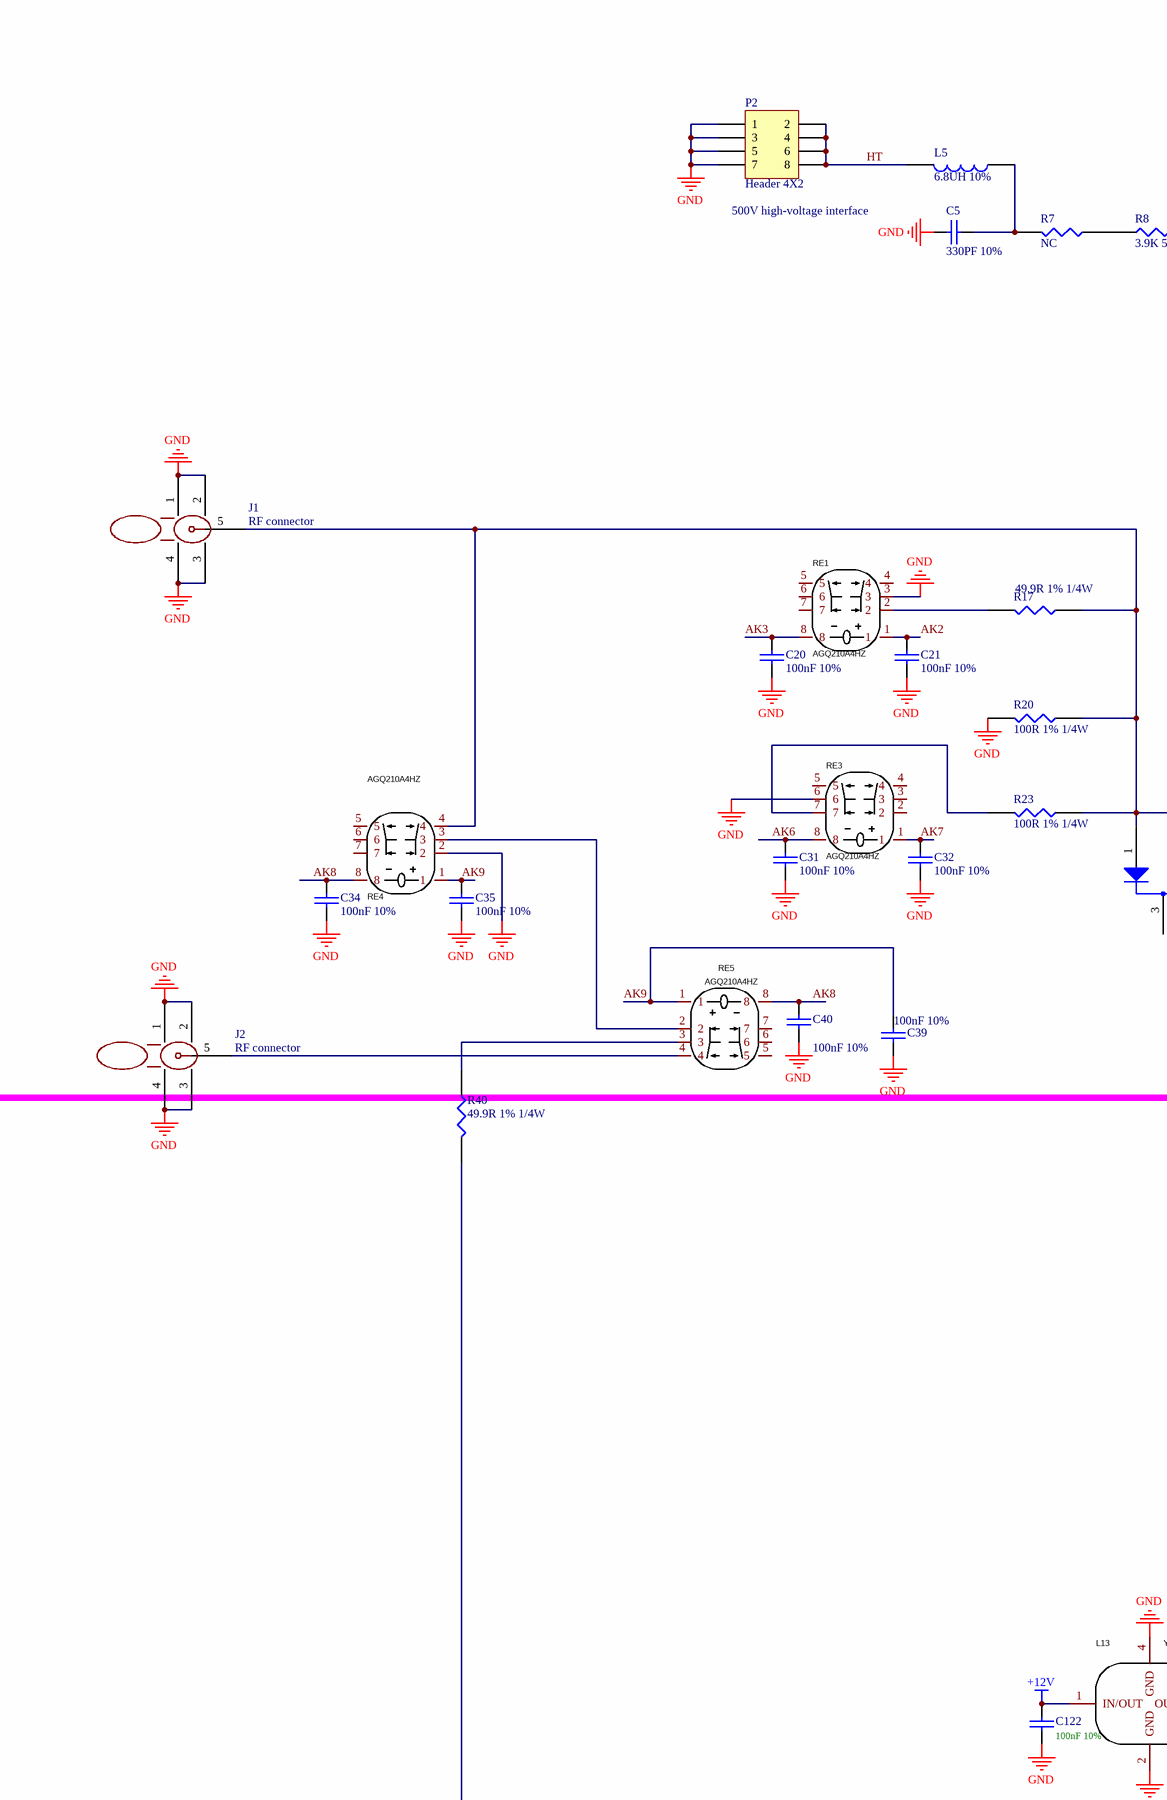
[diagram p0: PCBE109560-10.SchDoc, top left]
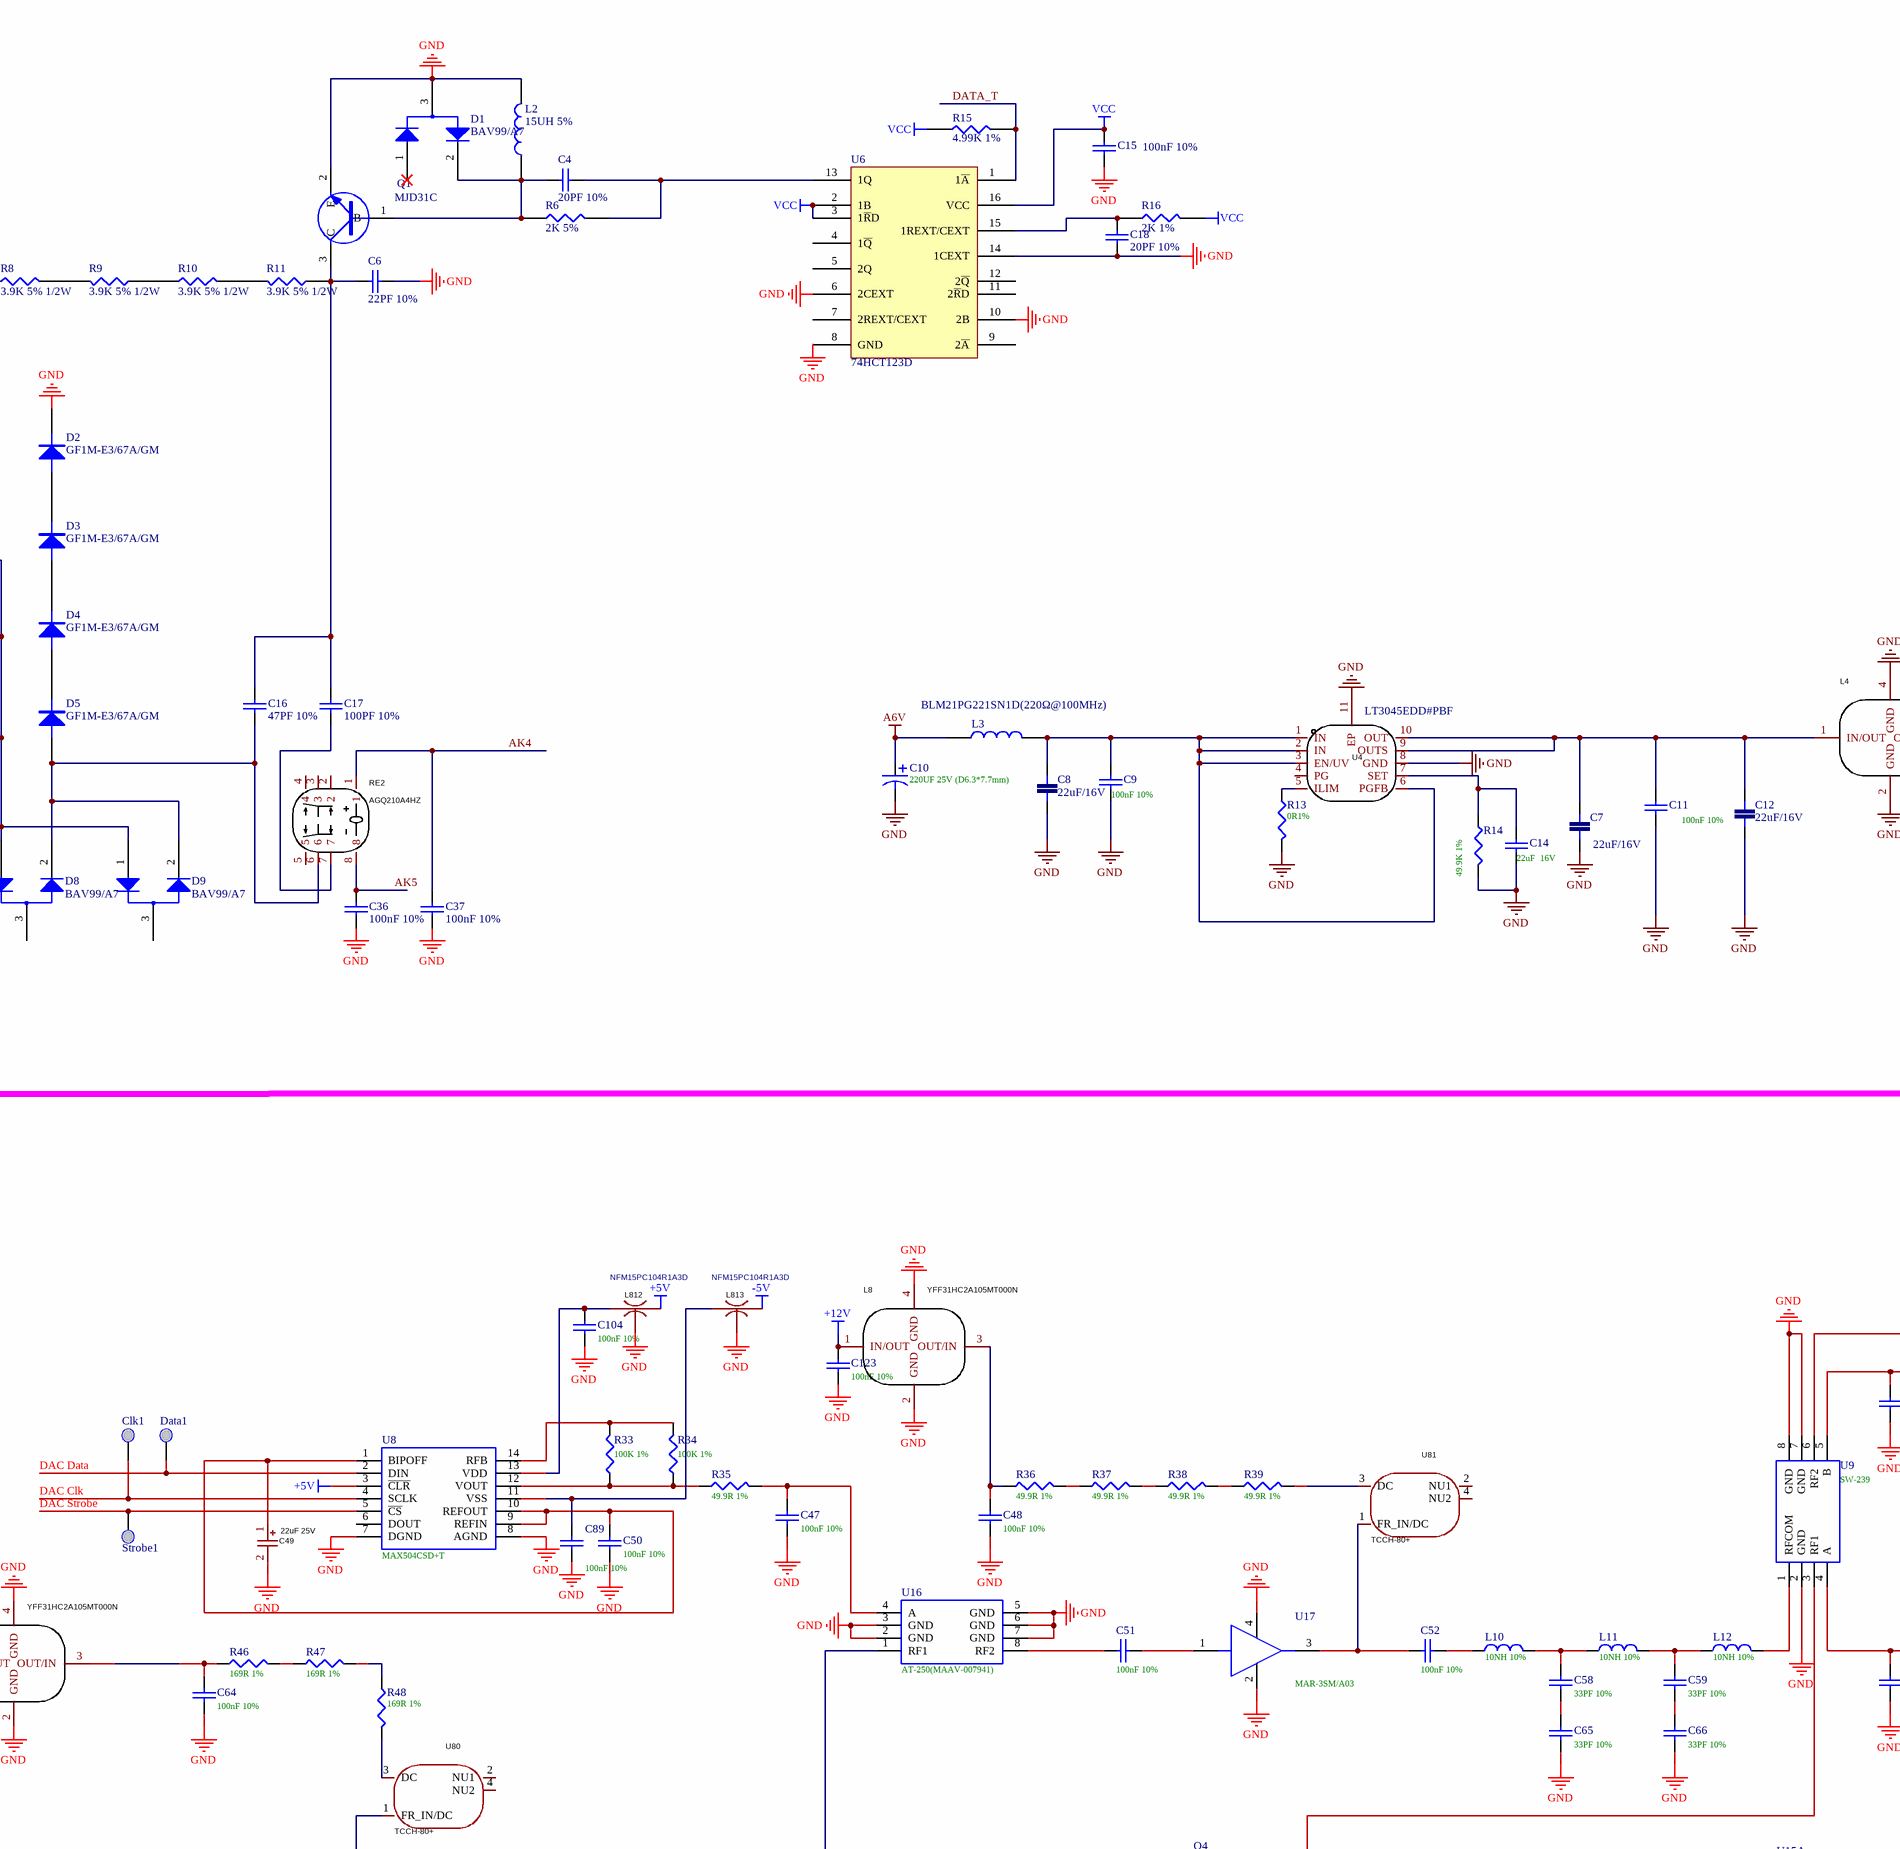
[diagram p1: PCBE109560-10.SchDoc, top middle]
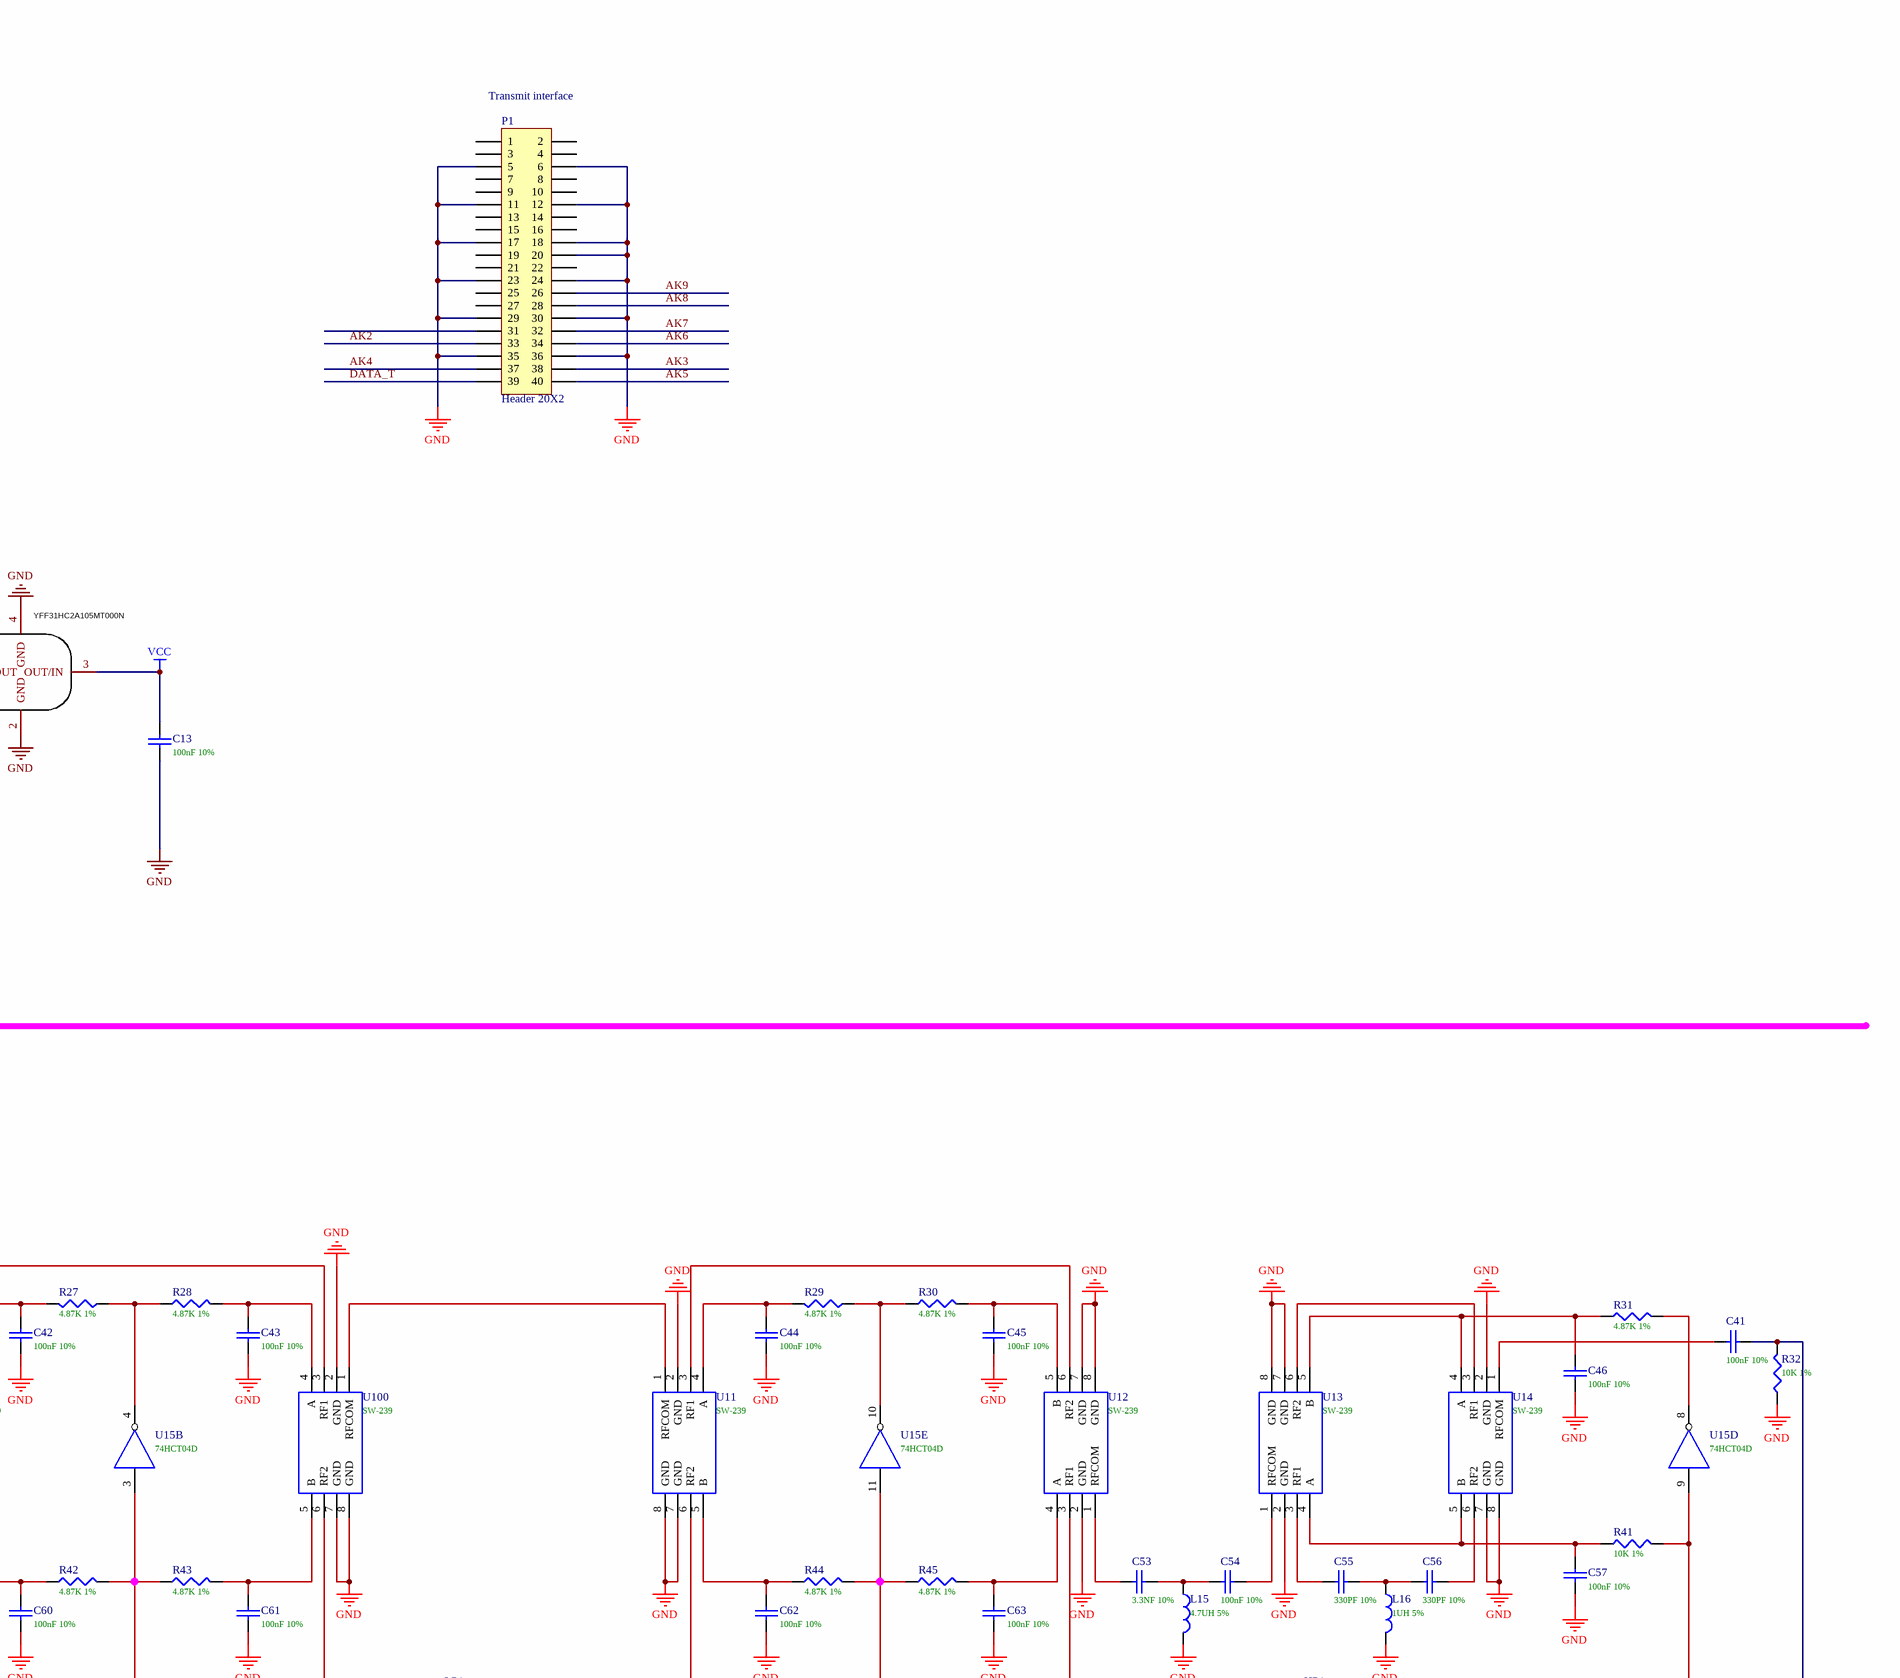
[diagram p2: PCBE109560-10.SchDoc, top right]
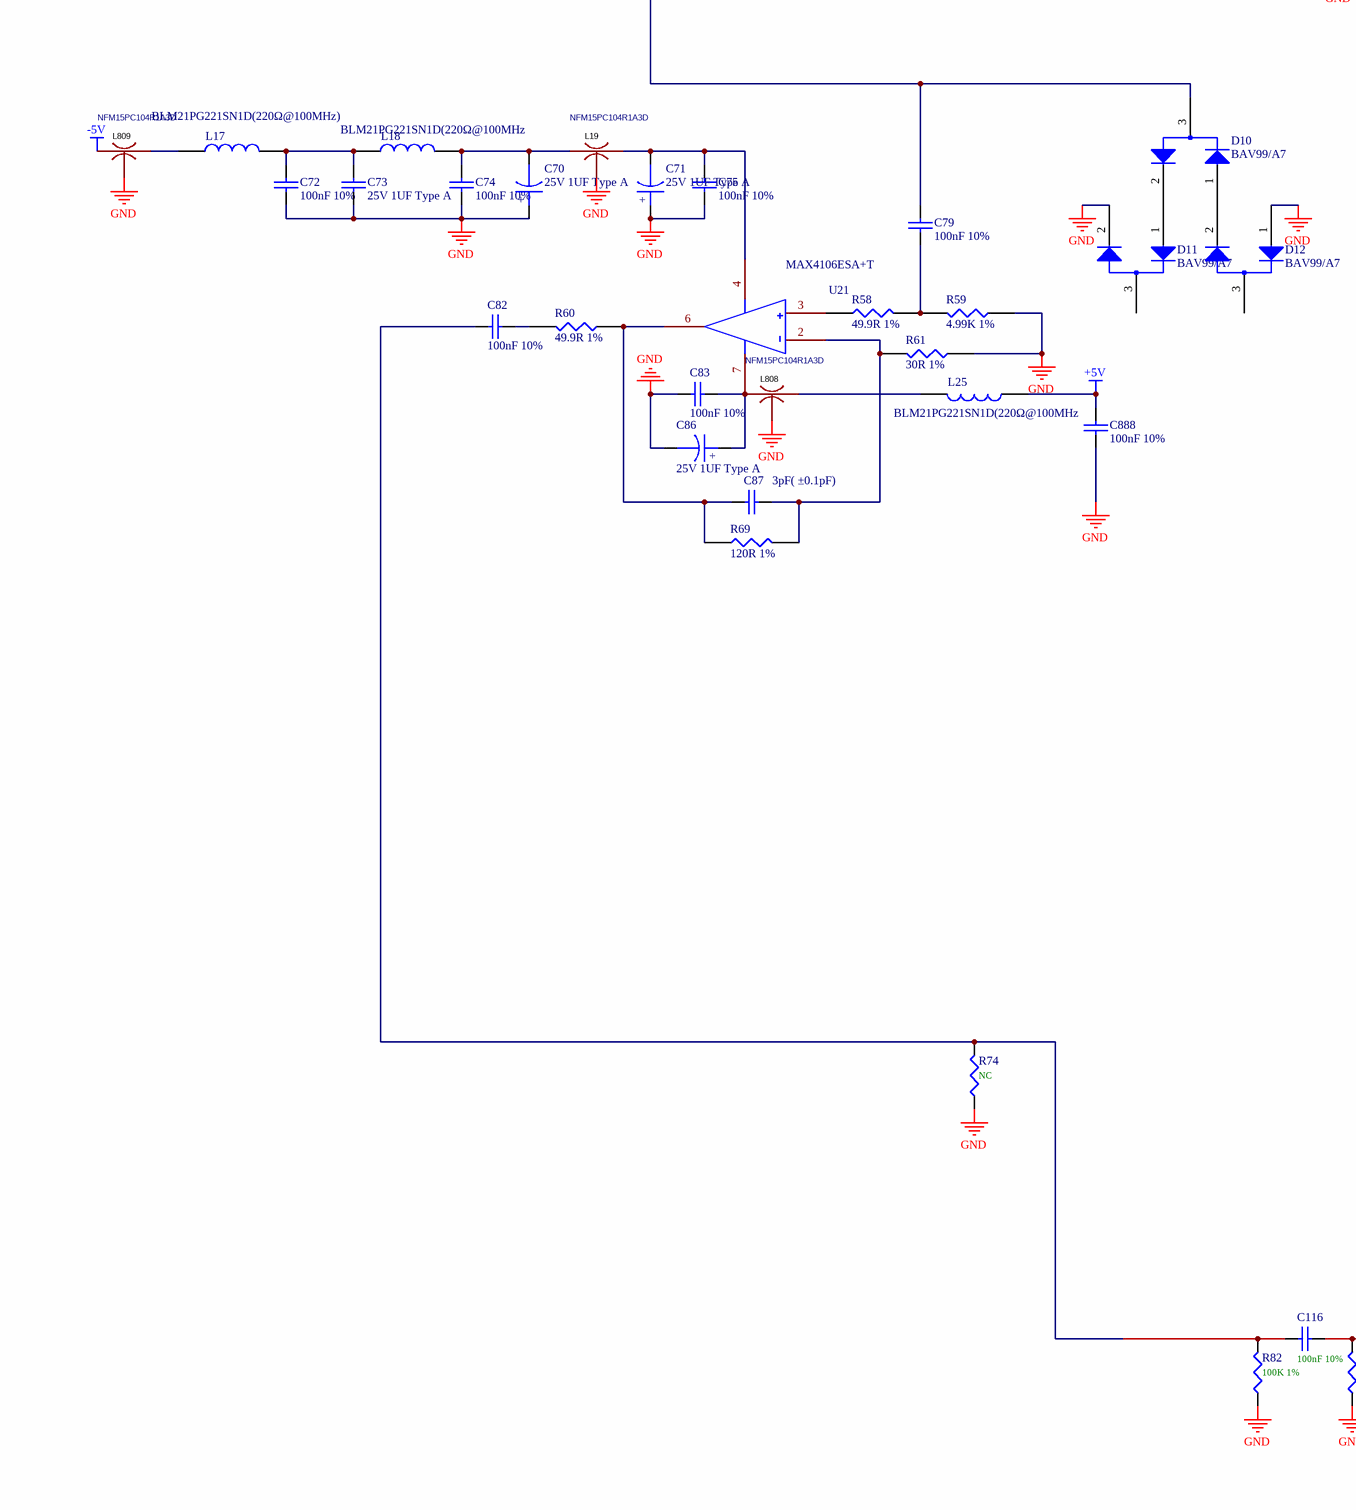
[diagram p3: PCBE109560-10.SchDoc, bottom left]
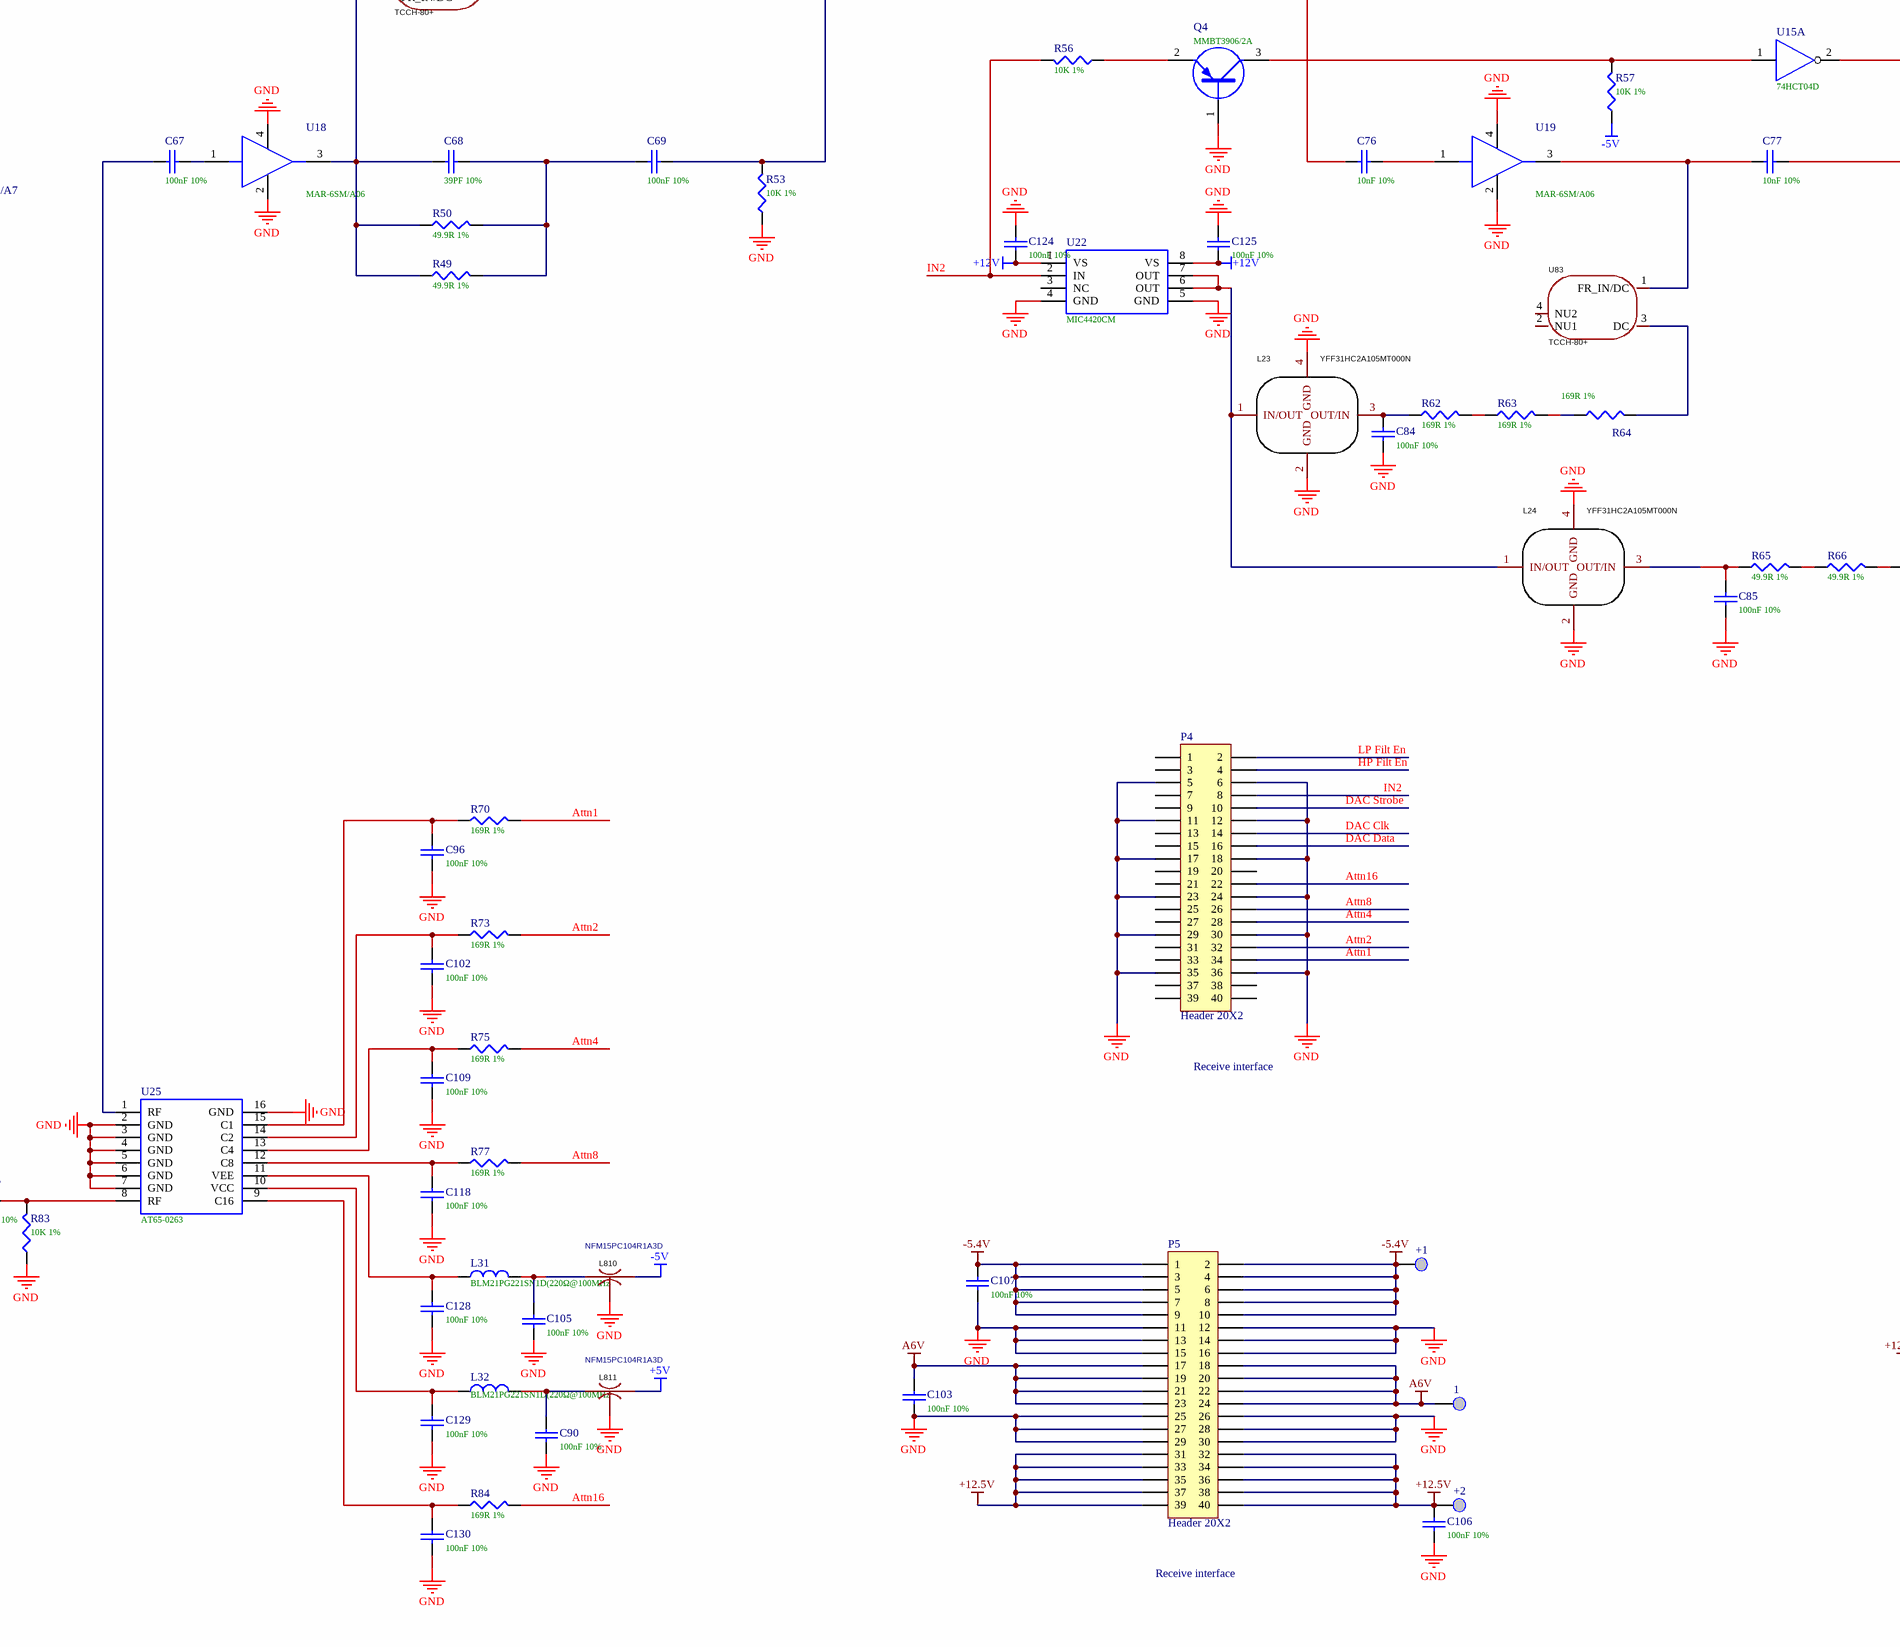
[diagram p4: PCBE109560-10.SchDoc, bottom middle]
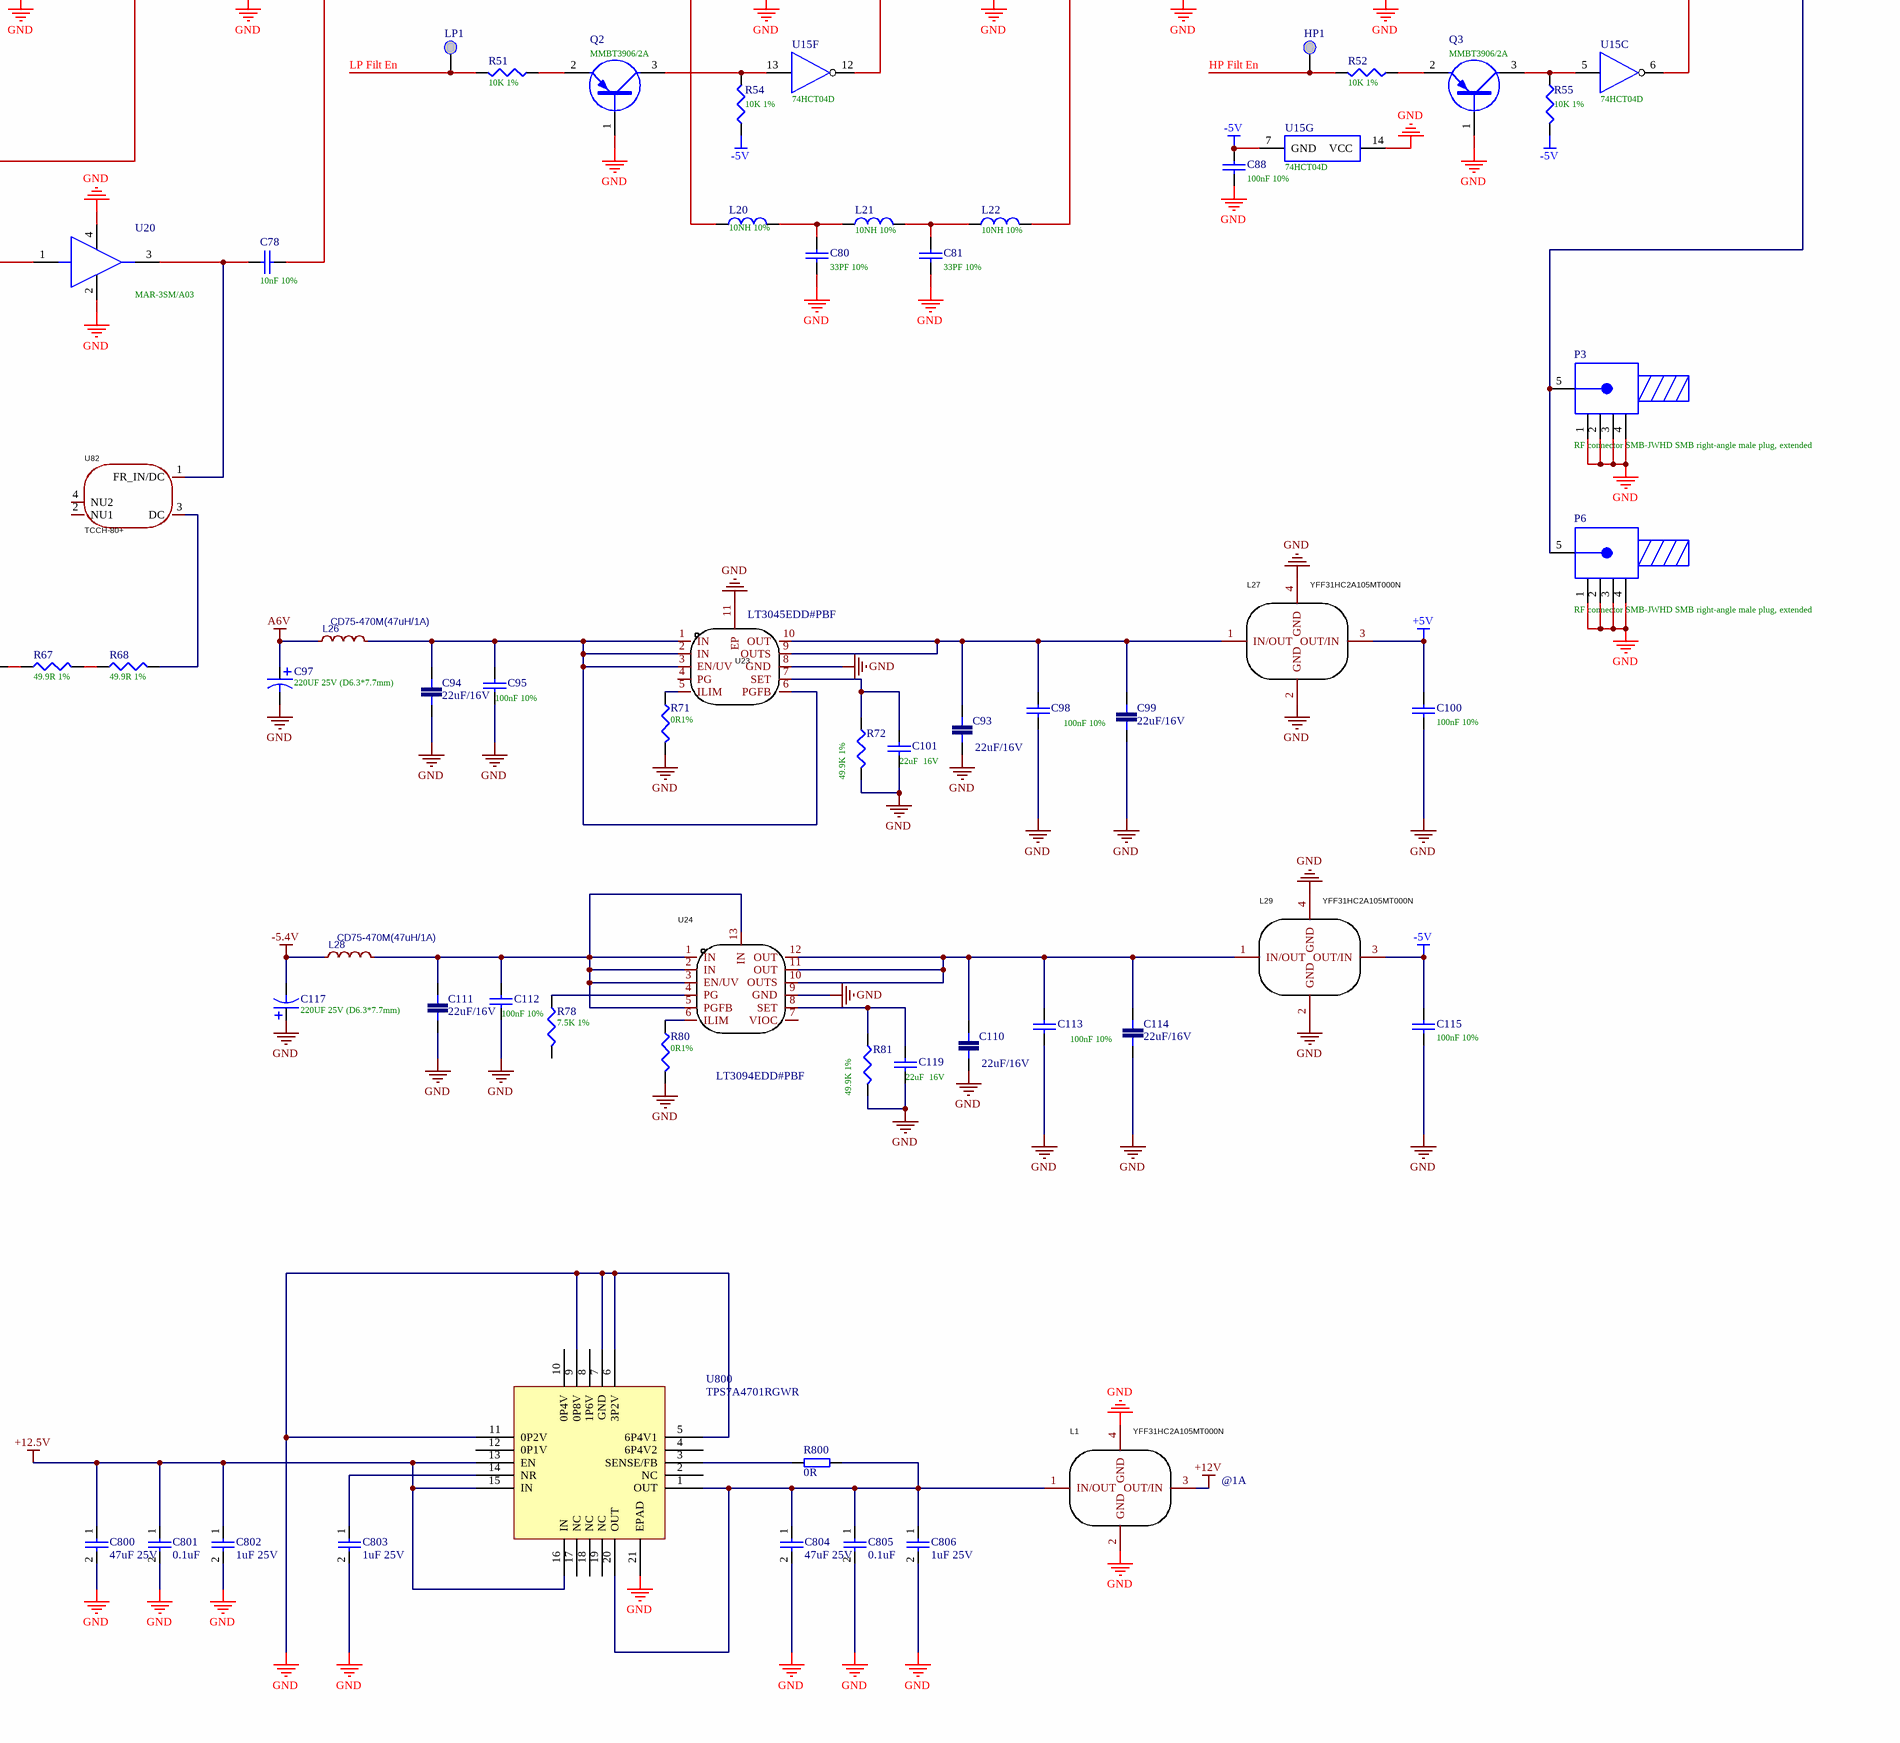
[diagram p5: PCBE109560-10.SchDoc, bottom right]
# Altium schematic sheet PCBE109560-10.SchDoc (part 1 of 2)
size E; SheetNumber: 0; SheetTotal: 0